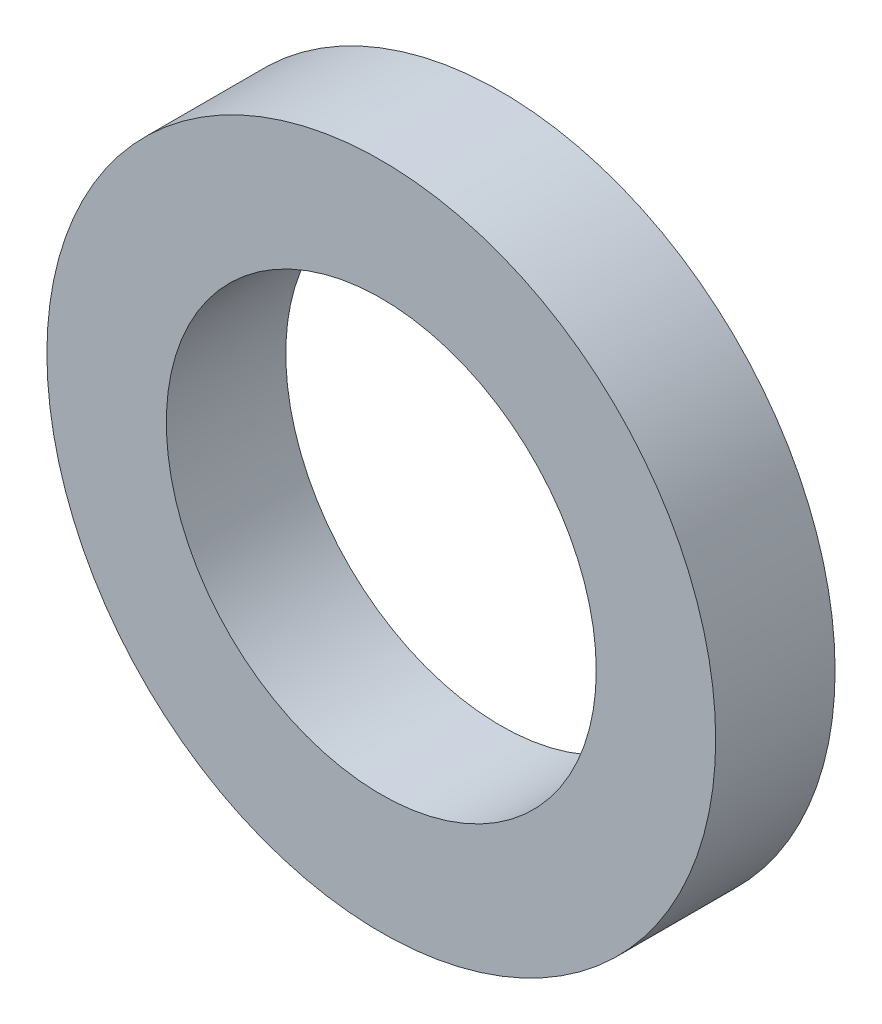
SolidWorks part; units mm, degrees
ref_plane "前视基准面" through (0, 0, 0) normal (0, 0, 1) x (1, 0, 0)
ref_plane "上视基准面" through (0, 0, 0) normal (0, 1, 0) x (1, 0, 0)
ref_plane "右视基准面" through (0, 0, 0) normal (1, 0, 0) x (0, 0, -1)
other "Configuration Table"
sketch "草图1" plane through (0, 0, 0) normal (0, 0, 1) x (1, 0, 0)
  circle A0 centre (0, 0) radius 140
  circle A1 centre (0, 0) radius 90
  point P0 (0, 0)
  dimension "D1" = 180
  dimension "D2" = 280
extrude "凸台-拉伸1" add sketch "草图1" against normal mid plane 50
